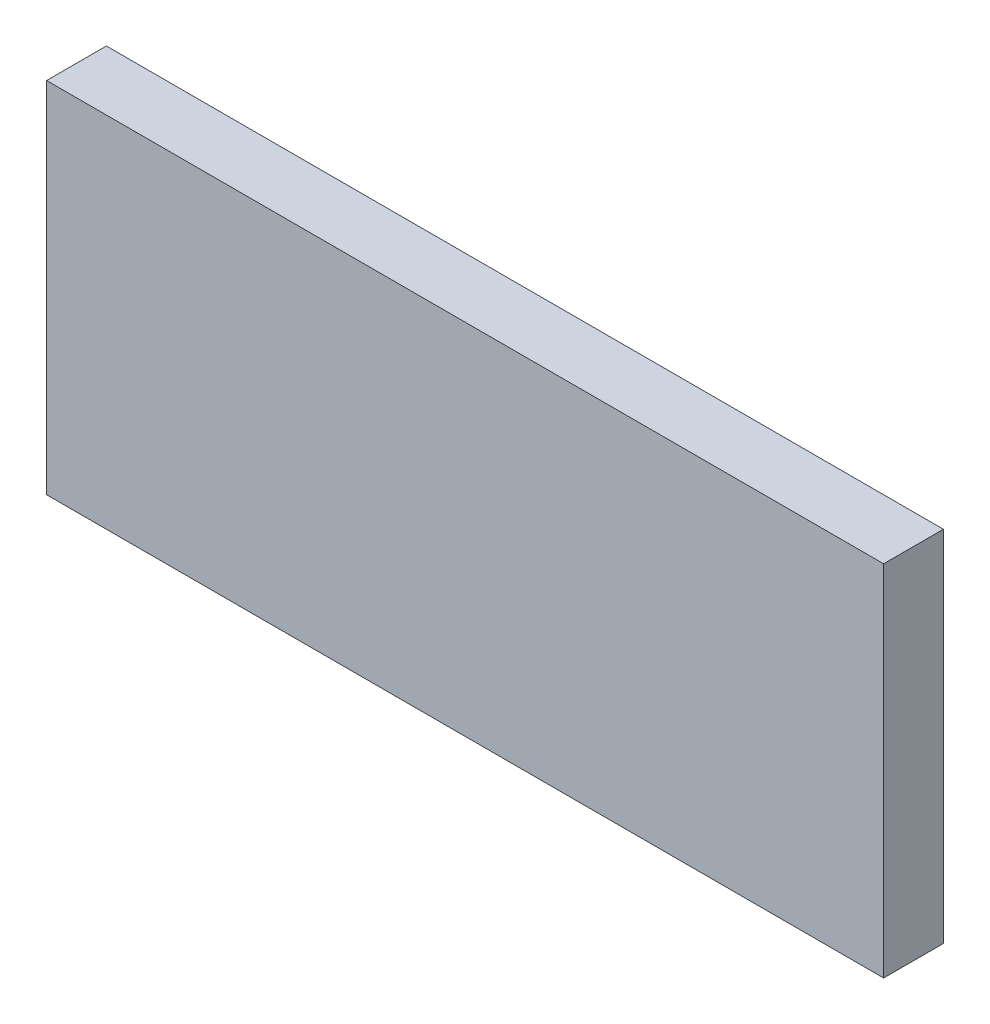
SolidWorks part; units mm, degrees
ref_plane "前视基准面" through (0, 0, 0) normal (0, 0, 1) x (1, 0, 0)
ref_plane "上视基准面" through (0, 0, 0) normal (0, 1, 0) x (1, 0, 0)
ref_plane "右视基准面" through (0, 0, 0) normal (1, 0, 0) x (0, 0, -1)
sketch "草图1" plane through (0, 0, 0) normal (0, 0, 1) x (1, 0, 0)
  line L0 (0, 0) -> (-140, 0)
  line L1 (-140, 60) -> (0, 60)
  line L2 (-140, 0) -> (-140, 60)
  line L3 (0, 60) -> (0, 0)
extrude "凸台-拉伸1" add sketch "草图1" along normal blind 10
